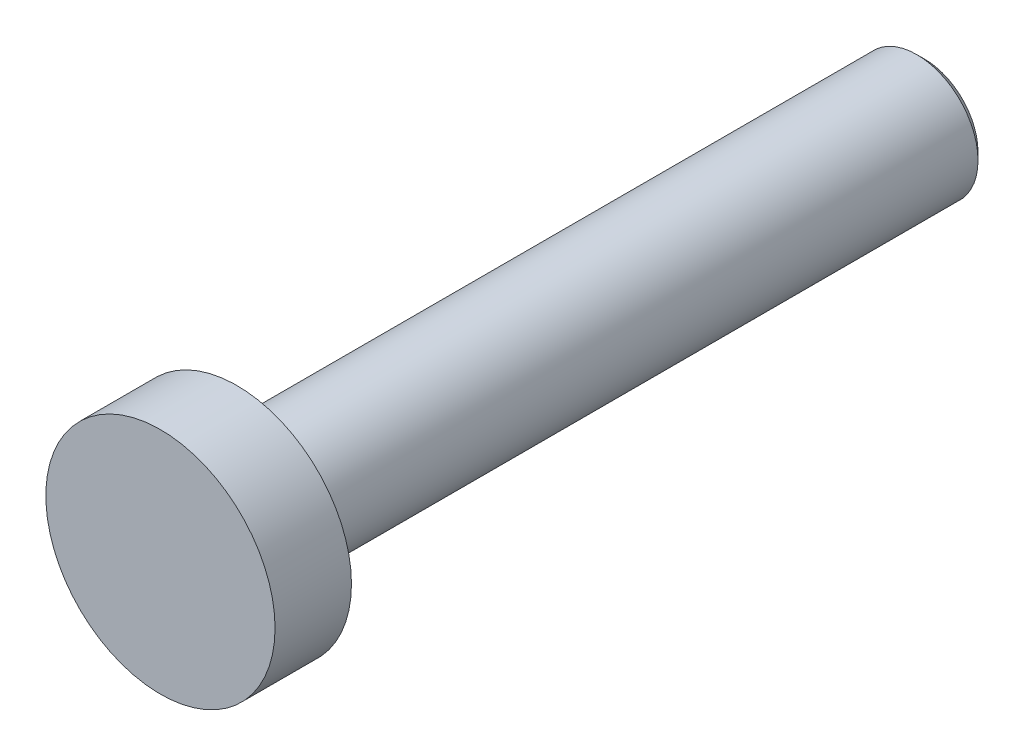
from build123d import *

# Parameters (mm, degrees)
SKETCH1_R           = 4
BOSS_EXTRUDE1_DEPTH = 45
SKETCH2_R           = 7.5
BOSS_EXTRUDE2_DEPTH = 5
CHAMFER1_SIZE       = 0.5


with BuildPart() as part:
    # Sketch1 → Boss-Extrude1 (new body)
    with BuildSketch(Plane.XY):
        with Locations(Location((0, 0, 0), (0, 0, 180))):
            Circle(SKETCH1_R)
    extrude(amount=BOSS_EXTRUDE1_DEPTH)

    # Sketch2 → Boss-Extrude2 (add)
    with BuildSketch(Plane.XY.offset(45)):
        Circle(SKETCH2_R)
    extrude(amount=BOSS_EXTRUDE2_DEPTH)

    # Chamfer1
    chamfer1_edges = [part.edges().sort_by_distance(p)[0] for p in [
        (4, 0, 0),
    ]]
    chamfer(chamfer1_edges, length=CHAMFER1_SIZE)


solid = part.part
